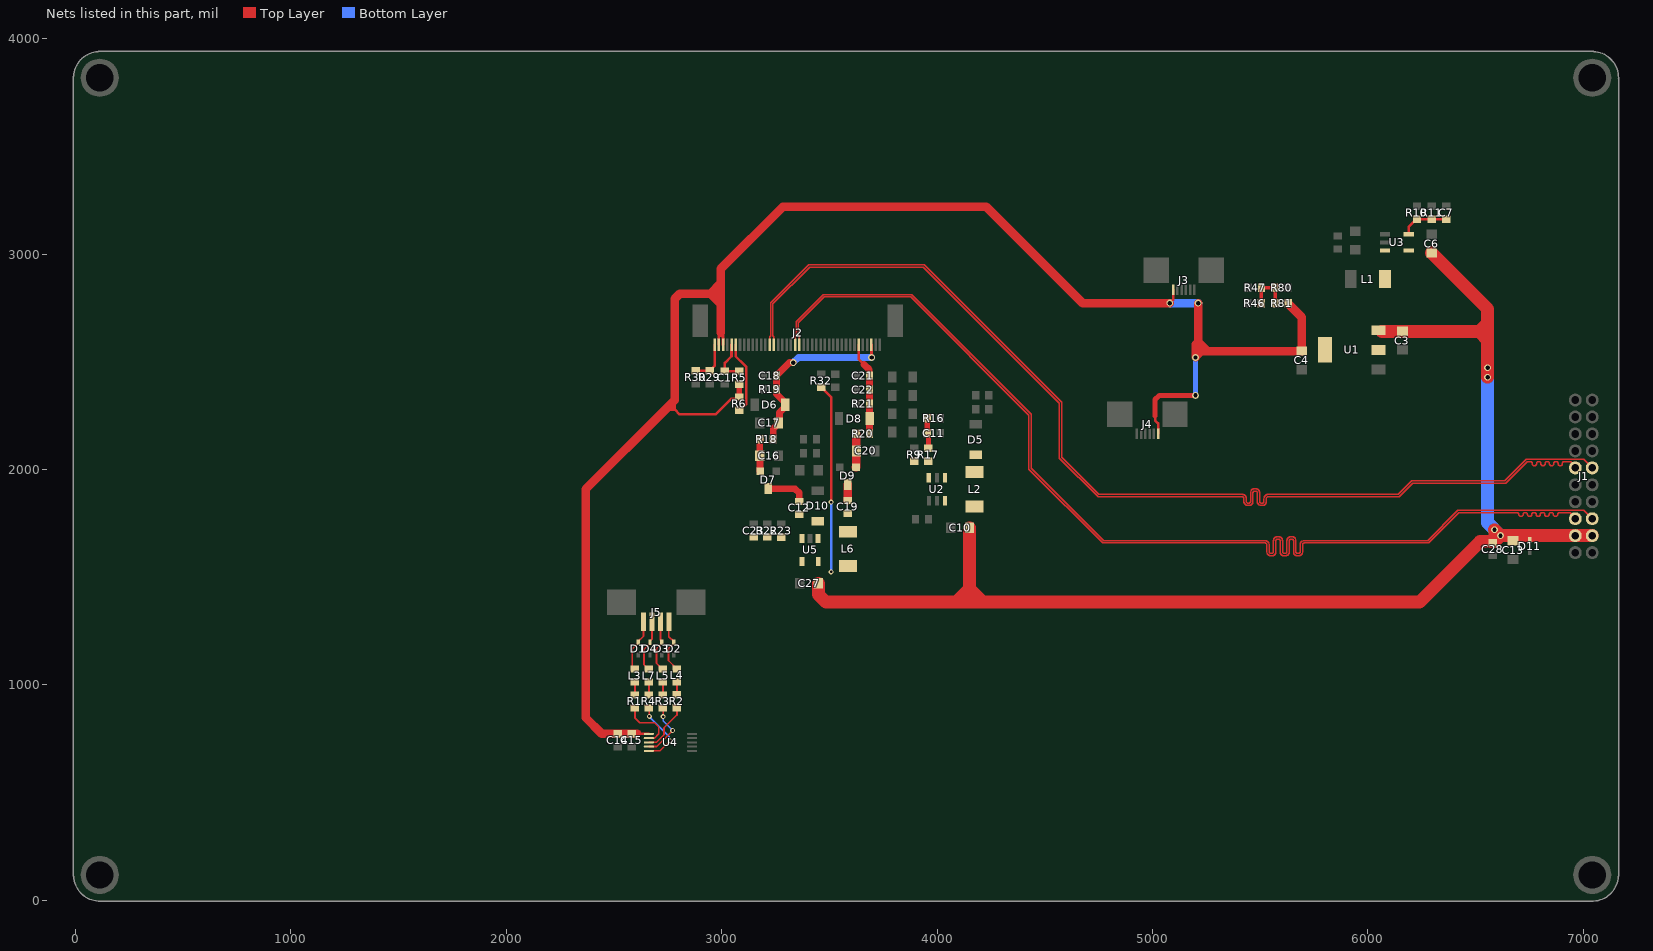
[diagram p0: the nets of this part, all layers, seen from the top]
# Altium PCB MISC82162.PcbDoc (part 3 of 3)
Units mil, origin at the board's own origin, x right, y up, seen from the top; angles counter-clockwise.
Board outline 7173.26 x 3944.91 mil, 2 copper layers (Top Layer, Bottom Layer); 90 components, 54 nets, 272 pads, 794 vias.
Unrouted connection lines stored in the file: 61.

## Via types
v1: diameter 23.62, hole 11.81, Top Layer to Bottom Layer, 779 vias
v2: diameter 32, hole 20, Top Layer to Bottom Layer, 13 vias
v3: diameter 31.5, hole 19.68, Top Layer to Bottom Layer, 2 vias

## Nets (pads, with @x,y where several pads share a name; then routed paths per layer and width w, separated by ;. In a path a pad name is that pad's centre, name@x,y a point inside that pad or via, vN(x,y) a via of type N, cw(c..) or ccw(c..) an arc to the next point about the centre after c; other vN are vias at no path point) (continued)
LVDS0-D2N: J1.10 J2.14 | length 4927.7
  Top Layer w6: J2.14@3222.67,2578.24 3222.67,2615.67 3227.01,2620.01 3227.01,2774.01 3403,2950 3939.56,2950 4578,2311.56 4578,2057.56 4751.56,1884 5377,1884 5416.5,1884 cw(c5416.5,1865) 5435.5,1865 5435.5,1851.68 ccw(c5443.5,1851.68) 5443.5,1843.68 5447.5,1843.68 ccw(c5447.5,1851.68) 5455.5,1851.68 5455.5,1891.62 cw(c5474.5,1891.62) 5474.5,1910.62 5478.5,1910.62 cw(c5478.5,1891.62) 5497.5,1891.62 5497.5,1851.68 ccw(c5505.5,1851.68) 5505.5,1843.68 5509.5,1843.68 ccw(c5509.5,1851.68) 5517.5,1851.68 5517.5,1865 cw(c5536.5,1865) 5536.5,1884 5581,1884 6141,1884 6203.35,1946.35 6634.79,1946.35 6735.69,2047.24 7001.69,2047.24 J1.10@7041.57,2007.37
LVDS0-D2P: J1.9 J2.15 | length 4925.6
  Top Layer w6: J2.15@3242.35,2578.24 3242.35,2615.65 3238.01,2619.99 3238.01,2769.46 3407.56,2939 3935,2939 4567,2307 4567,2053 4747,1873 5377,1873 5416.5,1873 cw(c5416.5,1865) 5424.5,1865 5424.5,1851.68 ccw(c5443.5,1851.68) 5443.5,1832.68 5447.5,1832.68 ccw(c5447.5,1851.68) 5466.5,1851.68 5466.5,1891.62 cw(c5474.5,1891.62) 5474.5,1899.62 5478.5,1899.62 cw(c5478.5,1891.62) 5486.5,1891.62 5486.5,1851.68 ccw(c5505.5,1851.68) 5505.5,1832.68 5509.5,1832.68 ccw(c5509.5,1851.68) 5528.5,1851.68 5528.5,1865 cw(c5536.5,1865) 5536.5,1873 5581,1873 6145.56,1873 6207.91,1935.35 6639.35,1935.35 6736,2032 6740.24,2036.24 6755,2036.24 cw(c6755,2028.24) 6763,2028.24 6763,2025.51 ccw(c6771,2025.51) 6771,2017.51 6775,2017.51 ccw(c6775,2025.51) 6783,2025.51 6783,2028.24 cw(c6791,2028.24) 6791,2036.24 6795,2036.24 cw(c6795,2028.24) 6803,2028.24 6803,2025.51 ccw(c6811,2025.51) 6811,2017.51 6815,2017.51 ccw(c6815,2025.51) 6823,2025.51 6823,2028.24 cw(c6831,2028.24) 6831,2036.24 6835,2036.24 cw(c6835,2028.24) 6843,2028.24 6843,2025.51 ccw(c6851,2025.51) 6851,2017.51 6855,2017.51 ccw(c6855,2025.51) 6863,2025.51 6863,2028.24 cw(c6871,2028.24) 6871,2036.24 6875,2036.24 cw(c6875,2028.24) 6883,2028.24 6883,2025.51 ccw(c6891,2025.51) 6891,2017.51 6895,2017.51 ccw(c6895,2025.51) 6903,2025.51 6903,2028.24 cw(c6911,2028.24) 6911,2036.24 6930.53,2036.24 6941.54,2036.24 6962.83,2014.96 J1.9@6962.83,2007.35
LVDS0-D3N: J1.16 J2.20 | length 4896.8
  Top Layer w6: J2.20@3340.78,2596.9 3340.78,2619.78 3345.12,2624.12 3345.12,2686.12 3471,2812 3882,2812 4437,2257 4437,2005.56 4772.78,1669.78 5483.25,1669.78 5522.75,1669.78 cw(c5522.75,1650.78) 5541.75,1650.78 5541.75,1617.78 ccw(c5549.75,1617.78) 5549.75,1609.78 5553.75,1609.78 ccw(c5553.75,1617.78) 5561.75,1617.78 5561.75,1668.62 cw(c5580.75,1668.62) 5580.75,1687.62 5584.75,1687.62 cw(c5584.75,1668.62) 5603.75,1668.62 5603.75,1617.78 ccw(c5611.75,1617.78) 5611.75,1609.78 5615.75,1609.78 ccw(c5615.75,1617.78) 5623.75,1617.78 5623.75,1668.62 cw(c5642.75,1668.62) 5642.75,1687.62 5646.75,1687.62 cw(c5646.75,1668.62) 5665.75,1668.62 5665.75,1617.78 ccw(c5673.75,1617.78) 5673.75,1609.78 5677.75,1609.78 ccw(c5677.75,1617.78) 5685.75,1617.78 5685.75,1650.78 cw(c5704.75,1650.78) 5704.75,1669.78 5729,1669.78 6277.78,1669.78 6418,1810 6420.28,1810 6421.22,1810.94 7001.77,1810.94 J1.16@7041.57,1771.15
LVDS0-D3P: J1.15 J2.21 | length 4904.5
  Top Layer w6: J2.21@3357.56,2593.99 3361,2597.43 3361,2619 3356.12,2623.88 3356.12,2681.57 3475.56,2801 3877.44,2801 4426,2252.44 4426,2001 4768.22,1658.78 5483.25,1658.78 5522.75,1658.78 cw(c5522.75,1650.78) 5530.75,1650.78 5530.75,1617.78 ccw(c5549.75,1617.78) 5549.75,1598.78 5553.75,1598.78 ccw(c5553.75,1617.78) 5572.75,1617.78 5572.75,1668.62 cw(c5580.75,1668.62) 5580.75,1676.62 5584.75,1676.62 cw(c5584.75,1668.62) 5592.75,1668.62 5592.75,1617.78 ccw(c5611.75,1617.78) 5611.75,1598.78 5615.75,1598.78 ccw(c5615.75,1617.78) 5634.75,1617.78 5634.75,1668.62 cw(c5642.75,1668.62) 5642.75,1676.62 5646.75,1676.62 cw(c5646.75,1668.62) 5654.75,1668.62 5654.75,1617.78 ccw(c5673.75,1617.78) 5673.75,1598.78 5677.75,1598.78 ccw(c5677.75,1617.78) 5696.75,1617.78 5696.75,1650.78 cw(c5704.75,1650.78) 5704.75,1658.78 5729,1658.78 6282.33,1658.78 6422.56,1799 6670,1799 6693,1799 cw(c6693,1791) 6701,1791 6701,1790.66 ccw(c6709,1790.66) 6709,1782.66 6713,1782.66 ccw(c6713,1790.66) 6721,1790.66 6721,1791.94 cw(c6729,1791.94) 6729,1799.94 6733,1799.94 cw(c6733,1791.94) 6741,1791.94 6741,1790.66 ccw(c6749,1790.66) 6749,1782.66 6753,1782.66 ccw(c6753,1790.66) 6761,1790.66 6761,1791.94 cw(c6769,1791.94) 6769,1799.94 6773,1799.94 cw(c6773,1791.94) 6781,1791.94 6781,1790.66 ccw(c6789,1790.66) 6789,1782.66 6793,1782.66 ccw(c6793,1790.66) 6801,1790.66 6801,1791.94 cw(c6809,1791.94) 6809,1799.94 6813,1799.94 cw(c6813,1791.94) 6821,1791.94 6821,1790.66 ccw(c6829,1790.66) 6829,1782.66 6833,1782.66 ccw(c6833,1790.66) 6841,1790.66 6841,1791.94 cw(c6849,1791.94) 6849,1799.94 6853,1799.94 cw(c6853,1791.94) 6861,1791.94 6861,1790.66 ccw(c6869,1790.66) 6869,1782.66 6873,1782.66 ccw(c6873,1790.66) 6881,1790.66 6881,1791 cw(c6889,1791) 6889,1799 6915,1799 6940.49,1799 6962.83,1776.67 J1.15@6962.83,1771.15
NetC7_2: C7.2 R10.1 R11.2 U3.5 | length 223.9
  Top Layer w12: U3.5@6189.62,3091.43 6189.62,3126.26 6225.05,3161.69 R10.1@6228,3161.69 R11.2@6296,3161.69 C7.2@6364,3161.69
NetC11_1: C11.1 R16.1 R17.2 | length 141.9
  Top Layer w24: R16.1@3954.03,2238.33 C11.1@3954.03,2168.33 3954.03,2165.38 3959.34,2160.07 R17.2@3959.34,2098.65
NetC12_1: C12.1 D7.3 | length 192.2
  Top Layer w32: D7.3@3216,1911 3216.93,1910.07 3341.26,1910.07 3360,1891.33 3360,1851.75 C12.1@3360.36,1851.39
NetC12_2: C12.2 C19.1 D10.1 L6.2 U5.1
NetC16_1: C16.1 D7.2 R18.1 | length 150.2
  Top Layer w32: R18.1@3177.68,2140 3177.68,2137.05 3176.69,2136.06 C16.1@3176.69,2064 3177.6,2063.1 3177.6,1991.9 D7.2@3178.5,1991
NetC19_2: C19.2 D9.3 | length 73.7
  Top Layer w40: C19.2@3585.36,1856.39 D9.3@3585.36,1930.07
NetC20_2: C20.2 D9.1 R20.1 | length 157.2
  Top Layer w40: D9.1@3622.86,2010.07 3623.71,2010.92 3623.71,2084.42 C20.2@3625.36,2086.07 3625.36,2165.76 R20.1@3625.05,2166.07
NetC23_2: C23.2 R22.1 R23.2 U5.3
NetD5_1: D5.1 L2.2 U2.1
NetJ2_6: J2.6 R6.2 | length 337.8
  Top Layer w12: J2.6@3065.19,2578.24 3065.19,2525.38 3105.34,2485.23 3113.29,2477.28 3113.29,2303.79 3084.65,2275.15 R6.2@3081.7,2275.15
NetL1_1: L1.1 U3.3
NetL3_2: L3.2 R1.1 | length 59.4
  Top Layer w8: R1.1@2597,953.32 L3.2@2597,1012.68
NetL4_2: L4.2 R2.1 | length 59.4
  Top Layer w8: R2.1@2792,953.83 L4.2@2792,1013.2
NetL5_2: L5.2 R3.1 | length 59.4
  Top Layer w8: R3.1@2727,953.32 L5.2@2727,1012.68
NetL7_2: L7.2 R4.1 | length 59.4
  Top Layer w8: R4.1@2662,953.32 L7.2@2662,1012.68
NetR1_2: R1.2 U4.2 | length 260.5
  Top Layer w8: R1.2@2597,892.68 2597,847 2620,824 2688,824 2708,804 2708,772.69 2688.35,753.04 2661.96,753.04 U4.2@2661.61,752.68
NetR2_2: R2.2 U4.3 | length 234.9
  Top Layer w8: U4.3@2661.61,733 2697,733 2732,768 2732,800 2792,860 R2.2@2792,893.2
NetR3_2: R3.2 U4.4 | length 264.7
  Top Layer w8: U4.4@2661.61,713.32 2661.96,713.67 2697.67,713.67 v1(2772,788) ; R3.2@2727,892.68 2728,891.68 v1(2728,852)
  Bottom Layer w8: v1(2728,852) 2728,832 v1(2772,788)
NetR4_2: R4.2 U4.5 | length 310.9
  Top Layer w8: U4.5@2661.61,693.63 2713.63,693.63 v1(2760,740) ; R4.2@2662,892.68 2664,890.68 v1(2664,853.72)
  Bottom Layer w8: v1(2664,853.72) 2664,852 2757.01,758.99 2757.01,742.99 v1(2760,740)
NetR9_2: R9.2 R17.1 U2.3
NetR46_1: R46.1 R47.1 R80.1 R81.2 | length 207.7
  Top Layer w16: R46.1@5504.7,2772.16 5505.51,2772.97 5505.51,2843.19 R47.1@5506.31,2844 5506.4,2844.08 5568.99,2844.08 R80.1@5569.07,2844.16 5569.38,2843.85 5569.38,2772.31 R81.2@5569.69,2772
RESET: C1.1 J2.5 R5.2 | length 199.8
  Top Layer w12: J2.5@3045.5,2578.24 3045.5,2525.5 3015,2495 C1.1@3015,2457 3015.21,2456.79 3080.52,2456.79 R5.2@3080.72,2456.59
VCC-3V3: C4.1 C14.1 C15.1 J2.2 J2.3 J3.1 J4.6 R5.1 R6.1 R81.1 U1.2 U1.4 U4.1 | length 8011.2
  Top Layer w12: 2606.68,773.32 2607.63,772.37 U4.1@2661.61,772.37 ; 2742,2282 2746,2278 2782,2278 ; 2760,2300 2782,2278 ; 2788,2328 2782,2322 2782,2278 ; J2.2@2986.45,2578.24 2986.45,2626.45 2996,2636 3006.13,2625.87 J2.3@3006.13,2578.24 ; R6.1@3081.7,2335.78 3073.93,2328.01 3044.01,2328.01 2972,2256 2804,2256 2782,2278 ; 5012,2248 5012,2228 5025.82,2214.18 J4.6@5025.82,2164.85 ; v2(5080,2772) 5080,2773.21 5095.82,2789.03 J3.1@5095.82,2833.94
  Top Layer w24: R5.1@3080.72,2395.96 3081.21,2395.47 3081.21,2336.27 R6.1@3081.7,2335.78 ; 5012,2248 5012,2324 5032,2344 v2(5200,2344)
  Top Layer w40: 2606.68,773.32 C15.1@2582,773.32 C14.1@2517,773.32 2442.68,773.32 2368,848 2368,1908 2742,2282 2760,2300 2782,2322 2782,2792.57 2805.43,2816 2948,2816 ; 2607.63,772.37 2608,772 ; 2996,2636 2996,2768 ; v2(5080,2772) 4676,2772 4228,3220 3284,3220 2996,2932 2996,2864 ; v2(5200,2520) v2@5200,2521.54 ; 5200,2549.54 5200,2540 ; 5212,2572 5212,2592 ; v2(5212,2772) 5212,2592 ; 5260,2549.54 5254.46,2549.54 ; R81.1@5630.31,2772 5630.31,2769.05 5692.46,2706.9 C4.1@5692.46,2549.54 5254.46,2549.54 ; 2948,2816 2996,2768 ; 2948,2816 2996,2816 ; 2948,2816 2996,2864 ; 2996,2768 2996,2816 ; 2996,2816 2996,2864 ; v2@5200,2521.54 5200,2540 ; v2@5200,2521.54 5228,2549.54 ; 5200,2540 5200,2580 5212,2592 ; 5200,2540 5209.54,2549.54 5228,2549.54 ; 5212,2592 5254.46,2549.54 ; 5228,2549.54 5254.46,2549.54
  Bottom Layer w24: v2(5200,2344) v2(5200,2520)
  Bottom Layer w40: v2(5080,2772) v2(5212,2772)
VCOM: J2.1 R29.1 R30.2 | length 195.1
  Top Layer w12: R30.2@2880,2458.32 2946.95,2458.32 2957.69,2469.05 2957.69,2472 2966.76,2481.08 2966.76,2548.27 J2.1@2966.76,2578.24
VDD5.0V: C3.1 C6.1 C10.1 C13.1 C27.1 C28.2 D11.1 J1.17 J1.18 L2.1 L6.1 R32.1 U1.3 U2.6 U3.4 U5.4 U5.5 | length 7507.6
  Top Layer w12: R32.1@3461.99,2381.59 3464.94,2381.59 3475.68,2370.86 3475.68,2367.91 3508,2335.59 v1(3508,1848)
  Top Layer w40: U1.3@6050.39,2645.92 6060.39,2645.92 6064.77,2641.54 C3.1@6160.46,2641.54
  Top Layer w60: C27.1@3448.67,1471.07 3448.67,1419.15 3483.82,1384 4088.15,1384 ; C10.1@4150.15,1729.43 4150.15,1446 ; 4236,1384 4212.15,1384 ; U1.3@6064.77,2641.54 6066.31,2640 C3.1@6160.46,2640 ; C3.1@6162,2640 6516,2640 ; C6.1@6296,3004.69 6556,2744.69 6556,2680 ; v2(6556,2428) v2(6556,2472) 6556,2600 ; v2(6588,1720) v2@6589,1719 ; J1.18@7041.57,1692.41 v2(6616.09,1692.41) ; 4088.15,1384 4150.15,1384 ; 4088.15,1384 4150.15,1446 ; 4150.15,1384 4212.15,1384 ; 4150.15,1384 4150.15,1446 ; 4150.15,1446 4212.15,1384 ; 4212.15,1384 6240,1384 6521.31,1665.32 C28.2@6589,1665.32 ; 6516,2640 6556,2600 ; 6516,2640 6556,2640 ; 6516,2640 6556,2680 ; 6556,2600 6556,2640 ; 6556,2640 6556,2680 ; C28.2@6589,1665.32 v2@6589,1719 ; C28.2@6589,1665.32 v2(6616.09,1692.41) ; v2@6589,1719 6615.59,1692.41 v2(6616.09,1692.41)
  Bottom Layer w12: v1(3508,1524) v1(3508,1848)
  Bottom Layer w60: v2(6556,2472) v2(6556,2428) 6556,1752.5 v2(6616.09,1692.41)
VGH: C17.1 C18.1 D6.2 J2.38 R18.2 R19.2 | length 873
  Top Layer w12: J2.38@3695.11,2578.24 3695.2,2578.14 3695.2,2520.8 v2(3696,2520)
  Top Layer w32: R18.2@3238.32,2140 3239.05,2140.73 3239.05,2188.39 3263.31,2212.65 C17.1@3263.31,2216 3268.96,2221.65 3268.96,2264.25 3294.87,2290.16 D6.2@3294.87,2300 3294.87,2309.84 3255.05,2349.66 3255.05,2371.27 R19.2@3254.32,2372 3254.32,2438.95 3255.05,2439.69 3258,2439.69 3314.32,2496 v2(3332,2496)
  Bottom Layer w32: v2(3332,2496) 3356,2520 v2(3696,2520)
VGL: C21.1 C22.1 D8.1 J2.35 R20.2 R21.2 | length 432.7
  Top Layer w12: J2.35@3636.06,2578.24 3636.06,2511.94 3660,2488
  Top Layer w32: 3660,2488 3684.94,2463.06 3684.94,2436.81 C21.1@3685.68,2436.07 C22.1@3685.68,2371.07 R21.2@3685.68,2306.07 R20.2@3685.68,2166.07
XN: D3.1 J5.3 L5.1 | length 246.3
  Top Layer w8: J5.3@2715.27,1292.31 2715.27,1208.19 2722,1201.46 D3.1@2722,1197.53 2722,1193.59 2697,1168.59 2697,1100.36 2724.05,1073.32 L5.1@2727,1073.32
XP: D1.1 J5.1 L3.1 | length 245.3
  Top Layer w8: L3.1@2597,1073.32 2585,1085.32 2585,1166.59 2612,1193.59 D1.1@2612,1197.53 2612,1201.46 2636.56,1226.02 J5.1@2636.56,1292.31
YN: D4.1 J5.2 L7.1 | length 245.5
  Top Layer w8: L7.1@2662,1073.32 2659.05,1073.32 2639,1093.36 2639,1165.59 2667,1193.59 D4.1@2667,1197.53 2667,1203 2675.92,1211.92 J5.2@2675.92,1292.31
YP: D2.1 J5.4 L4.1 | length 255.6
  Top Layer w8: J5.4@2754.64,1292.31 2754.64,1223.82 2777,1201.46 D2.1@2777,1197.53 2777,1193.59 2753,1169.59 2753,1112.83 2776.31,1089.51 2776.31,1086.56 2789.05,1073.83 L4.1@2792,1073.83
pads on no net: J2.4 J2.23 J2.24 J2.26 J2.27 J2.36 J2.37 J2.41 J2.42 J3.7 J3.8 J4.7 J4.8 J5.5 J5.6 VIA1.1 VIA2.1 VIA3.1 VIA4.1

## Polygon pours and split planes (outlines as drawn)
GND on Bottom Layer "GND_L02_P001" (solid, remove dead copper, pour order 1): 105.73,-4.27 cw(c112.43,117.61) -9.44,110.9 cw(c-5.68,112.09) -9.63,112.09 -9.63,3823.91 cw(c-5.68,3823.91) -9.44,3825.1 cw(c112.43,3818.39) 105.73,3940.27 cw(c106.92,3936.5) 106.92,3940.46 7047.22,3940.46 cw(c7047.22,3936.5) 7048.44,3940.26 cw(c7041.57,3818.39) 7163.63,3818.39 cw(c7041.57,3818.39) 7163.53,3813.49 cw(c7159.68,3812.61) 7163.63,3812.61 7163.63,111.96 cw(c7159.68,111.96) 7163.44,110.74 cw(c7041.57,117.61) 7036.66,-4.36 cw(c7035.79,-0.5) 7035.79,-4.46 106.92,-4.46 cw(c106.92,-0.5)
GND on Top Layer "GND_L01_P000" (solid, remove dead copper, pour order 0): 105.73,-4.27 cw(c112.43,117.61) -9.44,110.9 cw(c-5.68,112.09) -9.63,112.09 -9.63,3823.91 cw(c-5.68,3823.91) -9.44,3825.1 cw(c112.43,3818.39) 105.73,3940.27 cw(c106.92,3936.5) 106.92,3940.46 7047.22,3940.46 cw(c7047.22,3936.5) 7048.44,3940.26 cw(c7041.57,3818.39) 7163.63,3818.39 cw(c7041.57,3818.39) 7163.53,3813.49 cw(c7159.68,3812.61) 7163.63,3812.61 7163.63,111.96 cw(c7159.68,111.96) 7163.44,110.74 cw(c7041.57,117.61) 7036.66,-4.36 cw(c7035.79,-0.5) 7035.79,-4.46 106.92,-4.46 cw(c106.92,-0.5)

## Keep-outs
Keep-Out Layer:
  lines w7.87: -5.68,112.09 -5.68,3823.91 ; -5.54,123.25 ccw(c112.43,117.61) 106.78,-0.37 ; -5.54,3824.04 cw(c112.43,3818.39) 118.08,3936.37 ; 106.92,-0.5 7035.79,-0.5 ; 106.92,3936.5 7047.22,3936.5 ; 7035.92,-0.37 ccw(c7041.57,117.61) 7159.54,111.96 ; 7047.22,3936.37 cw(c7041.57,3818.39) 7159.54,3812.75 ; 7159.68,111.96 7159.68,3812.61

## Other copper
Top Layer:
  pour cut-out: 5912,2800 6092,2800 6088,2804 6088,2968 5916,2968 5912,2972
  pour cut-out: 4088,2000 4092,1996 4092,1820 4260,1820 4260,1996 4128,1996 4124,2000
  pour cut-out: 3500,1720 3500,1544 3672,1544 3672,1716 3500,1716 3496,1720
  region net LED9.3V: 3716,2588 3716,2552 3732,2536 3788,2536 3804,2552 3804,2588
  region net VDD5.0V: 6504,1644 6496,1652 6496,1684 6564,1752 6628,1752 6696,1684 6696,1644 6688,1644
  region net AVDD: 3412,1880 3412,2236 3388,2260 3388,2304 3416,2332 3428,2332 3480,2280 3480,1880
  region net NetC23_2: 3372,1704 3144,1704 3132,1692 3132,1644 3144,1632 3348,1632 3380,1664 3372,1672
  region net NetC12_2: 3444,1718 3364,1798 3364,1804 3376,1816 3604,1816 3628,1792 3628,1718
  region net NetC12_2: 3440,1772 3440,1672 3456,1656 3592,1656 3628,1692 3628,1744 3600,1772
  region net VDD5.0V: 3420,1440 3420,1504 3372,1552 3372,1592 3380,1600 3608,1600 3636,1572 3636,1524 3604,1492 3512,1492 3460,1440 3424,1440
  region net NetR9_2: 3968,1940 3904,1940 3876,1968 3876,2048 3976,2048 3976,1948
  region net NetD5_1: 4028,1940 4028,2000 4116,2088 4208,2088 4220,2076 4220,1968 4212,1960 4076,1960 4056,1940
  region net VDD5.0V: 4120,1692 4120,1784 4080,1824 4032,1824 4032,1876 4036,1880 4196,1880 4220,1856 4220,1732 4180,1692
  region net VCC-3V3: 6084,2532 5996,2532 5996,2432 5972,2408 5796,2408 5760,2444 5760,2508 5740,2528 5660,2528 5660,2652 5692,2684 5988,2684 5988,2596 6000,2584 6084,2584
  region net AVDD2.8V: 5948,2840 5888,2840 5888,2944 5827.91,3004.09 5827.91,3035.91 5832,3040 5968,3040 5968,2860
  region net NetL1_1: 6052,3024 6052,2856 6064,2844 6108,2844 6112,2848 6112,3012 6100,3024
  region net VDD5.0V: 6164,3028 6164,2968 6180,2952 6320,2952 6332,2964 6332,3024 6328,3028 6168,3028

## Silkscreen, mask and mechanical layers (free items; w line width, h text height)
Top Overlay:
  lines w5.91: 2577,1542.47 2577,3936.5 ; 2802,1543 2802,3936.5 ; 2937,2765.99 2937,3936.5 ; 3752,2765.99 3752,3936.5 ; 4910.14,2313.38 4910.14,3934.64 ; 5042.68,2313.38 5042.68,3935.82 ; 5077,2988 5077,3936.5 ; 5212,2987.49 5212,3933
  text "LCD_LVDS_7" at 940,889.99 h120
Bottom Overlay:
  lines w7.87: 332.91,-0.5 332.91,3936.5 6821.09,3936.5 6821.09,0.4 332.91,0.4